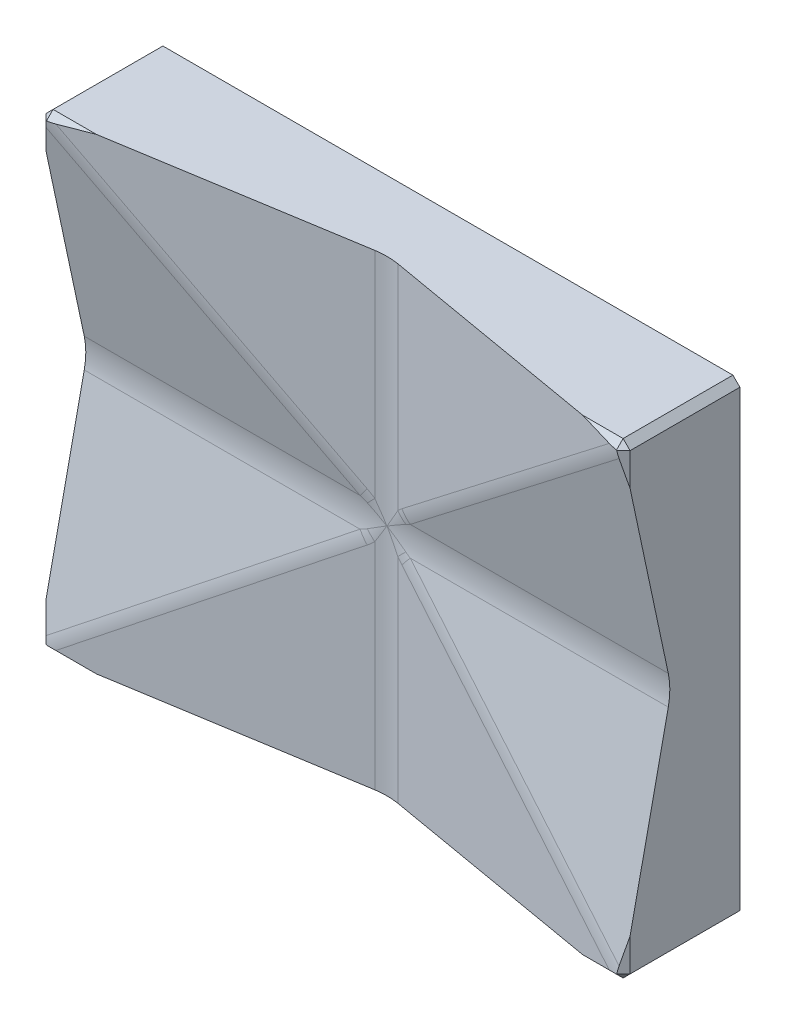
SolidWorks part; units mm, degrees
ref_plane "Front Plane" through (0, 0, 0) normal (0, 0, 1) x (1, 0, 0)
ref_plane "Top Plane" through (0, 0, 0) normal (0, 1, 0) x (1, 0, 0)
ref_plane "Right Plane" through (0, 0, 0) normal (1, 0, 0) x (0, 0, -1)
sketch "Sketch1" plane through (0, 0, 0) normal (0, 0, 1) x (1, 0, 0)
  line L1 (-12.5, 10) -> (12.5, 10)
  line L2 (-12.5, 10) -> (-12.5, -10)
  line L3 (-12.5, -10) -> (12.5, -10)
  line L4 (12.5, 10) -> (12.5, -10)
  line L5 (-12.5, 10) -> (12.5, -10) construction
  line L6 (-12.5, -10) -> (12.5, 10) construction
  point P0 (0, 0)
  dimension "D1" = 20
  dimension "D2" = 25
extrude "Boss-Extrude1" add sketch "Sketch1" along normal blind 5
chamfer "Chamfer1" distance 0.3 angle 45 8 edges at (0, -10, 5) (12.5, -10, 2.5) (12.5, 0, 5) (12.5, 10, 2.5) (0, 10, 5) (-12.5, 10, 2.5) (-12.5, 0, 5) (-12.5, -10, 2.5)
sketch "Sketch2" plane through (0, 10, 0) normal (0, 1, 0) x (1, 0, 0)
  line L0 (12.2, -5) -> (0.9011, -3.0439)
  line L2 (-0.0903, -3.0386) -> (-12.2, -5)
  line L4 (12.2, -5) -> (-12.2, -5)
  arc A0 (0.9011, -3.0439) -> (-0.0903, -3.0386) centre (0.3893, -6) ccw
  point P4 (0.4056, -3)
  dimension "D1" = 3
  dimension "D2" = 2
extrude "Cut-Extrude1" cut sketch "Sketch2" against normal up to next
sketch "Sketch3" plane through (-12.5, 0, 0) normal (-1, 0, 0) x (0, 0, 1)
  line L0 (5, 9.7) -> (3.0659, 0.6254)
  line L1 (3.0659, -0.6254) -> (5, -9.7)
  line L3 (5, -9.7) -> (5, 9.7)
  line L4 (5, 9.7) -> (5, -9.7) construction
  line L5 (5, -9.7) -> (4.7, -9.7) construction
  arc A0 (3.0659, 0.6254) -> (3.0659, -0.6254) centre (6, 0) ccw
  point P11 (3, 0)
  dimension "D1" = 3
  dimension "D2" = 2
extrude "Cut-Extrude2" cut sketch "Sketch3" against normal through all
fillet "Fillet1" radius 2 10 edges at (0.9614, -0.5685, 3.0544) (0.4087, -0.0105, 3) (0.9614, 0.5685, 3.0544) (-6.2296, 5.1627, 4.033) (-0.1692, 0.5525, 3.0513) (0.3729, 0.0026, 3) (-0.1692, -0.5525, 3.0513) (6.614, -5.1627, 4.033) (6.614, 5.1627, 4.033) (-6.2296, -5.1627, 4.033)
